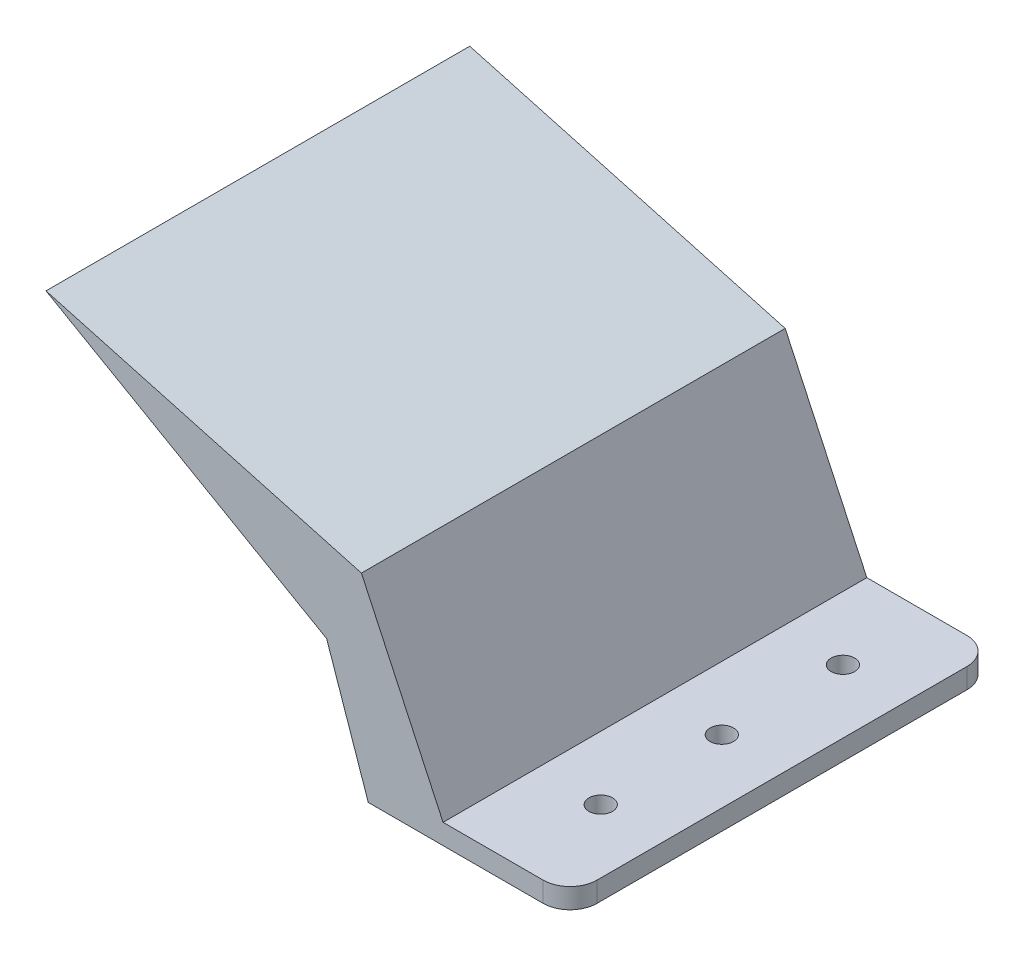
SolidWorks part; units mm, degrees
ref_plane "Front Plane" through (0, 0, 0) normal (0, 0, 1) x (1, 0, 0)
ref_plane "Top Plane" through (0, 0, 0) normal (0, 1, 0) x (1, 0, 0)
ref_plane "Right Plane" through (0, 0, 0) normal (1, 0, 0) x (0, 0, -1)
other "Configuration Table"
sketch "Sketch1" plane through (0, 0, 0) normal (0, 0, 1) x (1, 0, 0)
  line L0 (0, 0) -> (-6.1896, 18)
  line L1 (-6.1896, 18) -> (-47.9119, 41.9116)
  line L2 (-47.9119, 41.9116) -> (-1.0169, 29.025)
  line L3 (-1.0169, 29.025) -> (12.5176, 0)
  line L4 (12.5176, 0) -> (0, 0)
  dimension "D1" = 18
  dimension "D2" = 65
extrude "Boss-Extrude1" add sketch "Sketch1" along normal mid plane 63
sketch "Sketch2" plane through (0, 0, 31.5) normal (0, 0, 1) x (1, 0, 0)
  line L1 (0, 0) -> (30, 0)
  line L2 (0, 0) -> (0, 3)
  line L3 (0, 3) -> (30, 3)
  line L4 (30, 0) -> (30, 3)
  dimension "D1" = 3
  dimension "D2" = 30
extrude "Boss-Extrude2" add sketch "Sketch2" against normal up to surface (63 mm away) up to face at (-8.5202, 17.7873, -31.5)
sketch "Sketch3" plane through (0, 3, 0) normal (0, 1, 0) x (1, 0, 0)
  line L0 (20.5594, 31.5) -> (20.5594, -31.5) construction
  line L1 (30, 31.5) -> (11.1187, 31.5) construction
  line L2 (30, -31.5) -> (11.1187, -31.5) construction
  circle A0 centre (20.5594, 18.5) radius 1.75
  circle A1 centre (20.5594, 0.5) radius 1.75
  circle A2 centre (20.5594, -17.5) radius 1.75
  dimension "D1" = 3.5
  dimension "D2" = 13
  dimension "D4" = 18
  dimension "D3" = 3
extrude "Cut-Extrude1" cut sketch "Sketch3" against normal blind 50
fillet "Fillet1" radius 4 2 edges at (30, 1.5, 31.5) (30, 1.5, -31.5)
